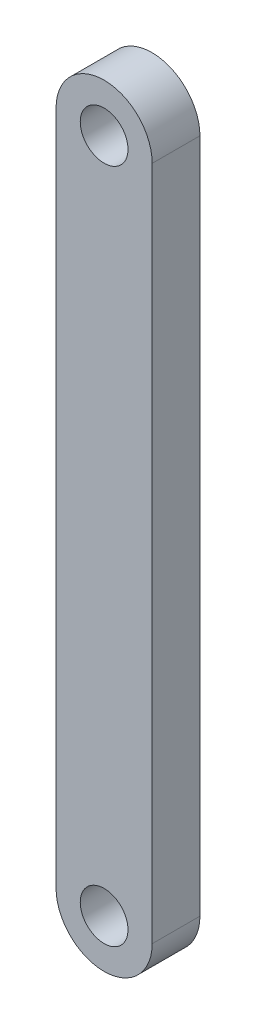
from build123d import *

# Parameters (mm, degrees)
SKETCH1_R           = 1.59
BOSS_EXTRUDE1_DEPTH = 3.18
SCALE_RATIO_1_SCALE = 1.3


with BuildPart() as part:
    # Sketch1 → Boss-Extrude1 (new body)
    with BuildSketch(Plane.XY):
        with BuildLine():
            Line((-3.2, 0), (-3.2, 45))
            ThreePointArc((-3.2, 45), (0, 48.2), (3.2, 45))
            Line((3.2, 45), (3.2, 0))
            ThreePointArc((3.2, 0), (0, -3.2), (-3.2, 0))
        make_face()
        with Locations(Location((0, 0, 0), (0, 0, 180))):
            Circle(SKETCH1_R, mode=Mode.SUBTRACT)
        with Locations(Location((0, 45, 0), (0, 0, 180))):
            Circle(SKETCH1_R, mode=Mode.SUBTRACT)
    extrude(amount=BOSS_EXTRUDE1_DEPTH)


with BuildPart() as part_1:
    # Scale ratio 1: scaled about (0, 0, 0)
    add(part.part.scale(SCALE_RATIO_1_SCALE))


solid = part_1.part
